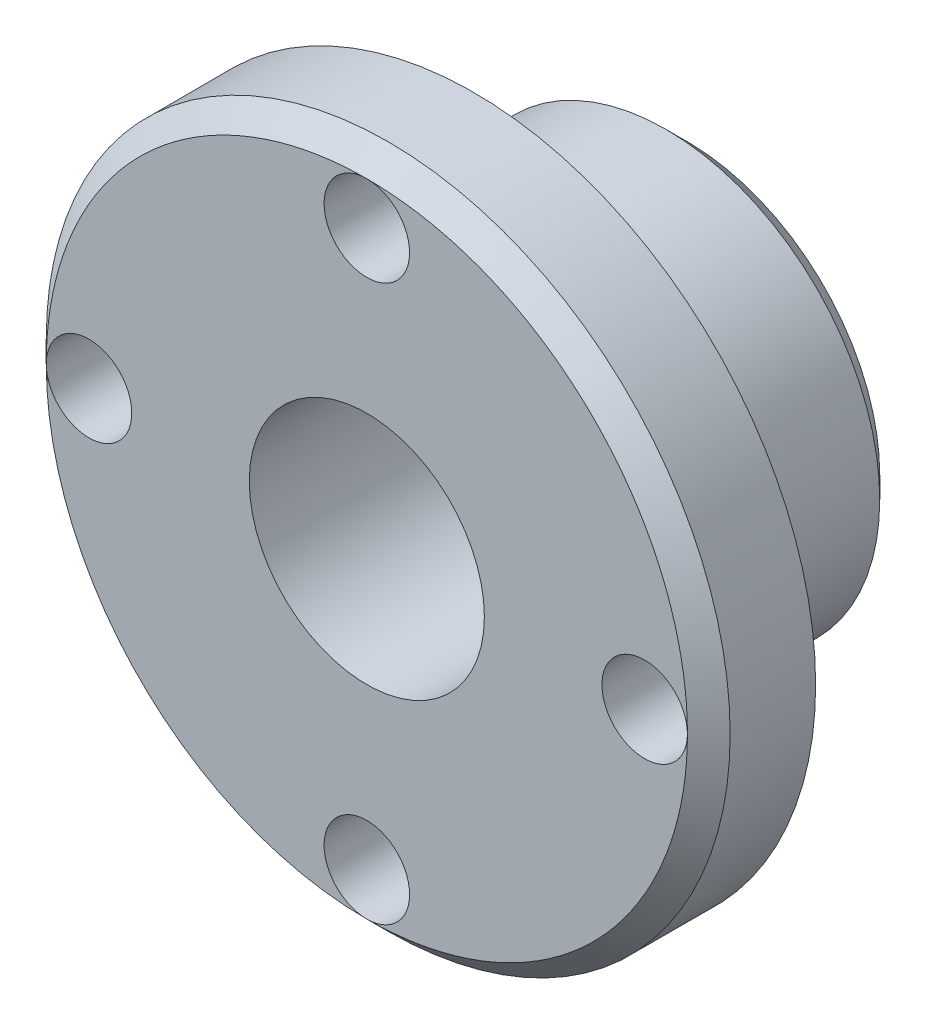
SolidWorks part; units mm, degrees
ref_plane "Front Plane" through (0, 0, 0) normal (0, 0, 1) x (1, 0, 0)
ref_plane "Top Plane" through (0, 0, 0) normal (0, 1, 0) x (1, 0, 0)
ref_plane "Right Plane" through (0, 0, 0) normal (1, 0, 0) x (0, 0, -1)
sketch "Sketch1" plane through (0, 0, 0) normal (0, 0, 1) x (1, 0, 0)
  circle A0 centre (0, 0) radius 10
  dimension "D1" = 20
extrude "Boss-Extrude1" add sketch "Sketch1" along normal blind 10
sketch "Sketch2" plane through (0, 0, 10) normal (0, 0, 1) x (1, 0, 0)
  circle A0 centre (0, 0) radius 16
  dimension "D1" = 32
extrude "Boss-Extrude2" add sketch "Sketch2" along normal blind 5
chamfer "Chamfer1" distance 1 angle 45 2 edges at (10, 0, 0) (16, 0, 15)
sketch "Sketch3" plane through (0, 0, 10) normal (0, 0, -1) x (-1, 0, 0)
  circle A1 centre (0, 13) radius 2
  dimension "D2" = 4
extrude "Cut-Extrude1" cut sketch "Sketch3" against normal blind 10
pattern_circular "CirPattern1" count 4 over 360 about axis through (0, 0, 0) along (0, 0, 1) of "Cut-Extrude1"
sketch "Sketch4" plane through (0, 0, 0) normal (0, 0, -1) x (-1, 0, 0)
  circle A0 centre (0, 0) radius 5.5
  dimension "D1" = 11
extrude "Cut-Extrude2" cut sketch "Sketch4" against normal blind 29
